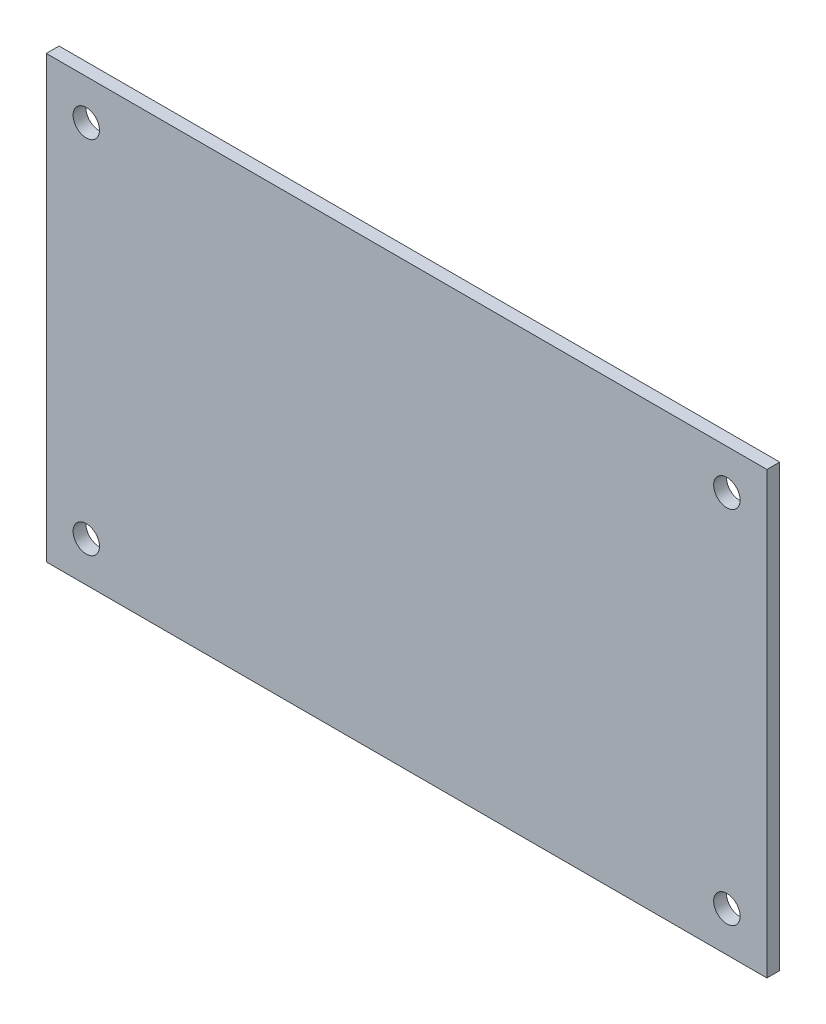
SolidWorks part; units mm, degrees
ref_plane "前视基准面" through (0, 0, 0) normal (0, 0, 1) x (1, 0, 0)
ref_plane "上视基准面" through (0, 0, 0) normal (0, 1, 0) x (1, 0, 0)
ref_plane "右视基准面" through (0, 0, 0) normal (1, 0, 0) x (0, 0, -1)
other "Configuration Table"
sketch "草图1" plane through (0, 0, 0) normal (0, 0, 1) x (1, 0, 0)
  line L0 (-45, -27.5) -> (45, -27.5)
  line L1 (45, -27.5) -> (45, 27.5)
  line L2 (45, 27.5) -> (-45, 27.5)
  line L3 (-45, 27.5) -> (-45, -27.5)
  circle A0 centre (-40, -22.5) radius 1.65
  circle A1 centre (-40, 22.5) radius 1.65
  circle A2 centre (40, -22.5) radius 1.65
  circle A3 centre (40, 22.5) radius 1.65
  point P0 (0, 0)
  dimension "D1" = 3.3
  dimension "D2" = 3.3
  dimension "D3" = 3.3
  dimension "D4" = 3.3
  dimension "D5" = 5
  dimension "D6" = 45
  dimension "D7" = 85
  dimension "D8" = 90
  dimension "D9" = 5
  dimension "D10" = 27.5
  dimension "D11" = 50
  dimension "D12" = 55
extrude "凸台-拉伸1" add sketch "草图1" against normal mid plane 1.6
